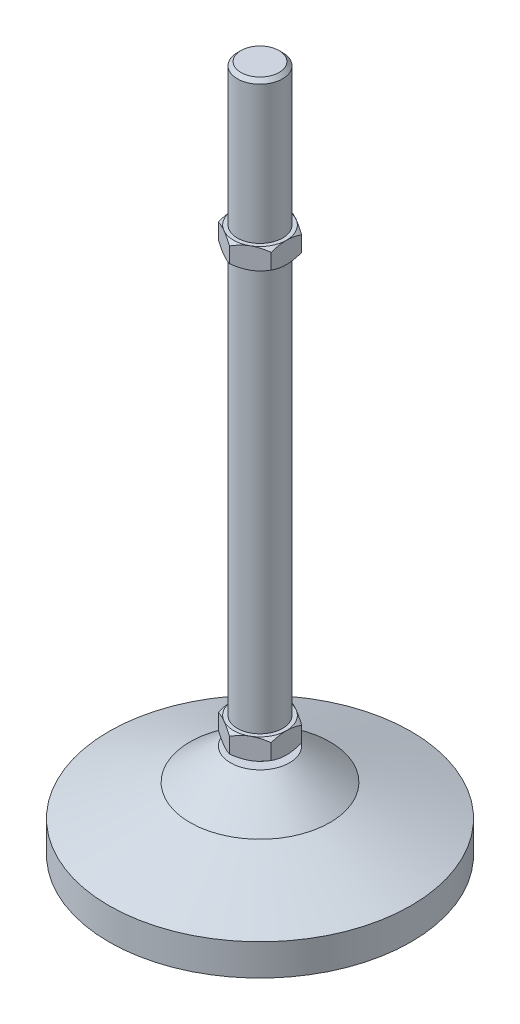
from build123d import *

# Parameters (mm, degrees)
CHAMFER1_SIZE       = 0.96
BOSS_EXTRUDE1_START = 26.4
BOSS_EXTRUDE1_DEPTH = 5.6
BOSS_EXTRUDE2_START = 138.9
BOSS_EXTRUDE2_DEPTH = 5.6
SKETCH6_R           = 9.165807537
SKETCH6_R_2         = 7
CUT_EXTRUDE4_DEPTH  = 5.6
CUT_EXTRUDE4_TAPER  = 55
SKETCH7_R           = 9.165807537
SKETCH7_R_2         = 7
CUT_EXTRUDE5_DEPTH  = 5.6
CUT_EXTRUDE5_TAPER  = 55
SKETCH9_R           = 9.165807537
SKETCH9_R_2         = 7
CUT_EXTRUDE6_DEPTH  = 5.6
CUT_EXTRUDE6_TAPER  = 55
SKETCH10_R          = 9.165807537
SKETCH10_R_2        = 7
CUT_EXTRUDE7_DEPTH  = 5.6
CUT_EXTRUDE7_TAPER  = 55


with BuildPart() as part:
    # Sketch2 → Revolve1 (revolve)
    with BuildSketch(Plane(origin=(0, 0, 0), x_dir=(0, 0, -1), z_dir=(1, 0, 0)), mode=Mode.PRIVATE) as revolve1_sk:
        Polygon((4.8, 32), (4.8, 25), (7.8, 25), (18.533333333, 16.666666667), (40, 8.333333333), (40, 0), (0, 0), (0, 182), (6, 182), (6, 32), align=None)
    revolve(revolve1_sk.sketch.rotate(Axis((0, 182, 0), (0, -1, 0)), 180), axis=Axis((0, 182, 0), (0, -1, 0)))

    # Chamfer1
    chamfer1_edges = [part.edges().sort_by_distance(p)[0] for p in [
        (0, 182, -6),
    ]]
    chamfer(chamfer1_edges, length=CHAMFER1_SIZE)


with BuildPart() as body_2:
    # Sketch3 → Boss-Extrude1 (new body)
    with BuildSketch(Plane(origin=(0, 0, 0), x_dir=(1, 0, 0), z_dir=(0, 1, 0)).offset(BOSS_EXTRUDE1_START)):
        Polygon((7, -4.041451884), (7, 4.041451884), (0, 8.082903769), (-7, 4.041451884), (-7, -4.041451884), (0, -8.082903769), align=None)
    extrude(amount=BOSS_EXTRUDE1_DEPTH)

    # Sketch6 → Cut-Extrude4 (cut)
    with BuildSketch(Plane(origin=(0, 32, 0), x_dir=(1, 0, 0), z_dir=(0, 1, 0))):
        Circle(SKETCH6_R)
        Circle(SKETCH6_R_2, mode=Mode.SUBTRACT)
    extrude(amount=-CUT_EXTRUDE4_DEPTH, taper=CUT_EXTRUDE4_TAPER, mode=Mode.SUBTRACT)

    # Sketch7 → Cut-Extrude5 (cut)
    with BuildSketch(Plane.XZ.offset(-26.4)):
        Circle(SKETCH7_R)
        Circle(SKETCH7_R_2, mode=Mode.SUBTRACT)
    extrude(amount=-CUT_EXTRUDE5_DEPTH, taper=CUT_EXTRUDE5_TAPER, mode=Mode.SUBTRACT)


with BuildPart() as body_3:
    # Sketch8 → Boss-Extrude2 (new body)
    with BuildSketch(Plane(origin=(0, 0, 0), x_dir=(1, 0, 0), z_dir=(0, 1, 0)).offset(BOSS_EXTRUDE2_START)):
        Polygon((7, -4.041451884), (7, 4.041451884), (0, 8.082903769), (-7, 4.041451884), (-7, -4.041451884), (0, -8.082903769), align=None)
    extrude(amount=BOSS_EXTRUDE2_DEPTH)

    # Sketch9 → Cut-Extrude6 (cut)
    with BuildSketch(Plane(origin=(0, 144.5, 0), x_dir=(1, 0, 0), z_dir=(0, 1, 0))):
        Circle(SKETCH9_R)
        Circle(SKETCH9_R_2, mode=Mode.SUBTRACT)
    extrude(amount=-CUT_EXTRUDE6_DEPTH, taper=CUT_EXTRUDE6_TAPER, mode=Mode.SUBTRACT)

    # Sketch10 → Cut-Extrude7 (cut)
    with BuildSketch(Plane.XZ.offset(-138.9)):
        Circle(SKETCH10_R)
        Circle(SKETCH10_R_2, mode=Mode.SUBTRACT)
    extrude(amount=-CUT_EXTRUDE7_DEPTH, taper=CUT_EXTRUDE7_TAPER, mode=Mode.SUBTRACT)


solid = Compound([part.part, body_2.part, body_3.part])
